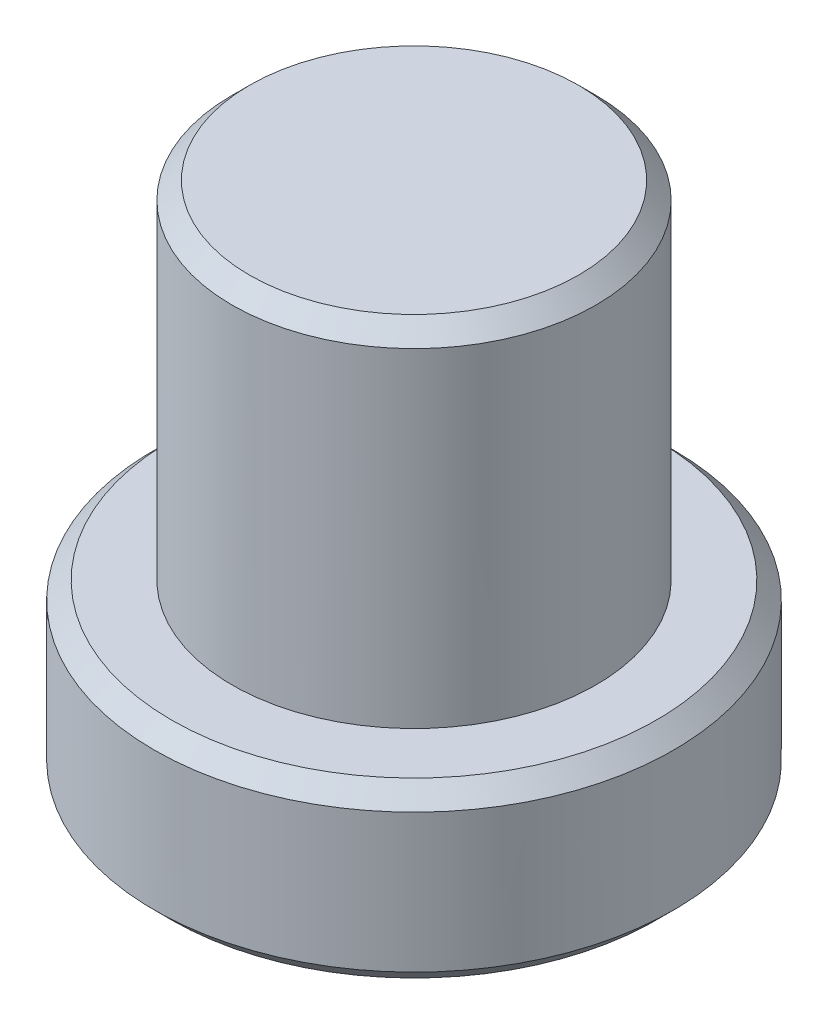
from build123d import *

# Parameters (mm, degrees)
CHAMFER1_SIZE = 0.5


with BuildPart() as part:
    # Sketch1 → Revolve1 (revolve)
    with BuildSketch(Plane(origin=(0, 0, 0), x_dir=(0, 0, -1), z_dir=(1, 0, 0))):
        Polygon((0, 15), (5.25, 15), (5.25, 5), (7.5, 5), (7.5, 0), (0, 0), align=None)
    revolve(axis=Axis((0, 0, 0), (0, 1, 0)))

    # Chamfer1
    chamfer1_edges = [part.edges().sort_by_distance(p)[0] for p in [
        (0, 0, 7.5),
        (0, 5, 7.5),
        (0, 15, 5.25),
    ]]
    chamfer(chamfer1_edges, length=CHAMFER1_SIZE)


solid = part.part
